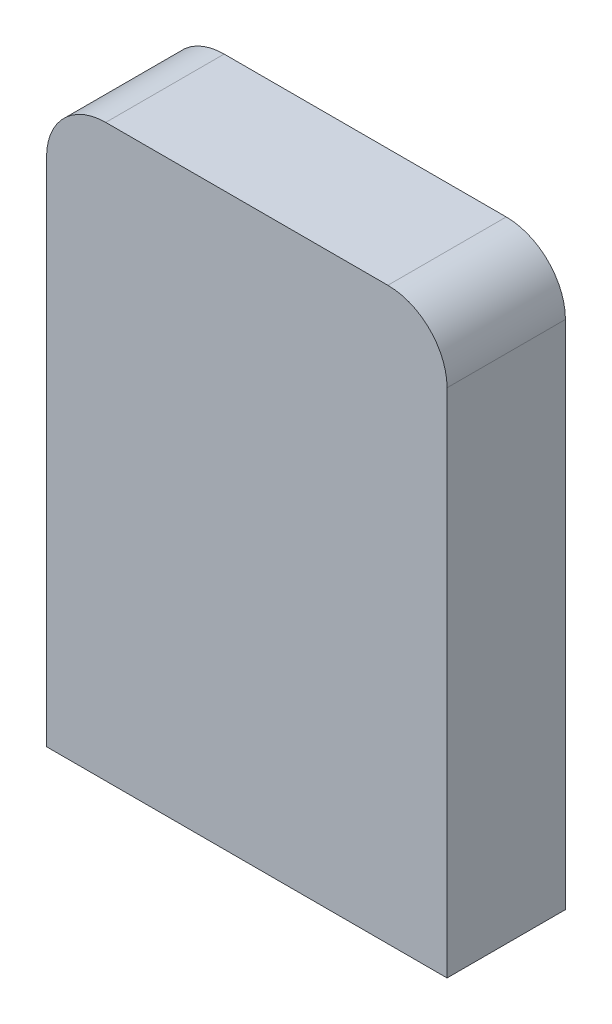
SolidWorks part; units mm, degrees
ref_plane "Front Plane" through (0, 0, 0) normal (0, 0, 1) x (1, 0, 0)
ref_plane "Top Plane" through (0, 0, 0) normal (0, 1, 0) x (1, 0, 0)
ref_plane "Right Plane" through (0, 0, 0) normal (1, 0, 0) x (0, 0, -1)
sketch "Sketch1" plane through (0, 0, 0) normal (0, 0, 1) x (1, 0, 0)
  line L8 (-11.5926, -51.9419) -> (22.7304, -51.9419)
  line L9 (22.7304, -51.9419) -> (22.7304, -76.7532)
  line L10 (22.7304, -76.7532) -> (92.1707, -76.7532)
  line L11 (92.1707, -76.7532) -> (92.1707, -51.9419)
  line L12 (92.1707, -51.9419) -> (123.7392, -51.9419)
  line L13 (123.7392, -51.9419) -> (123.7392, 120.7811)
  line L14 (103.7392, 140.7811) -> (8.4074, 140.7811)
  line L15 (-11.5926, 120.7811) -> (-11.5926, -51.9419)
  line L16 (-11.5926, -51.9419) -> (92.1707, -51.9419)
  line L20 (92.1707, -51.9419) -> (123.7392, -51.9419)
  line L21 (123.7392, -51.9419) -> (123.7392, 120.7811)
  line L22 (103.7392, 140.7811) -> (8.4074, 140.7811)
  line L23 (-11.5926, 120.7811) -> (-11.5926, -51.9419)
  arc A2 (123.7392, 120.7811) -> (103.7392, 140.7811) centre (103.7392, 120.7811) ccw
  arc A3 (8.4074, 140.7811) -> (-11.5926, 120.7811) centre (8.4074, 120.7811) ccw
  arc A4 (123.7392, 120.7811) -> (103.7392, 140.7811) centre (103.7392, 120.7811) ccw
  arc A5 (8.4074, 140.7811) -> (-11.5926, 120.7811) centre (8.4074, 120.7811) ccw
  dimension "D1" = 0
extrude "Boss-Extrude1" add sketch "Sketch1" along normal blind 40
shell "Shell1" thickness 5
